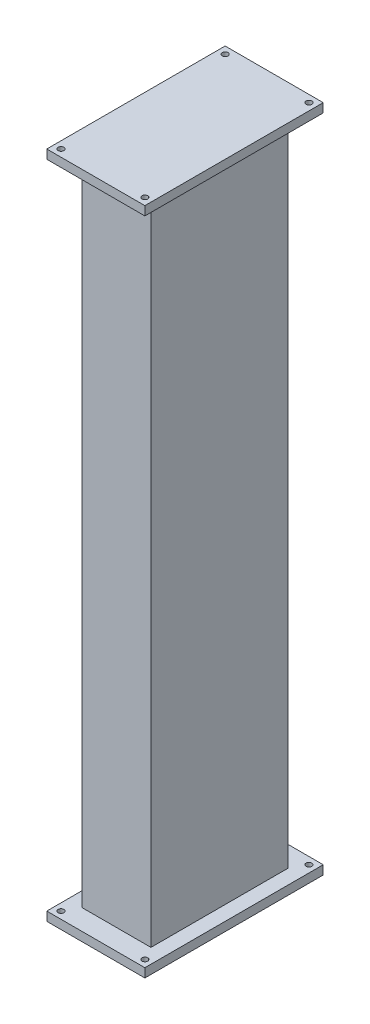
from build123d import *

# Parameters (mm, degrees)
SKETCH1_W           = 110
SKETCH1_H           = 200
SKETCH1_R           = 3.25
BOSS_EXTRUDE1_DEPTH = 10
SKETCH2_W           = 77.344894784
SKETCH2_H           = 153.75567248
BOSS_EXTRUDE2_DEPTH = 730
SKETCH4_W           = 110
SKETCH4_H           = 200
SKETCH4_R           = 3.25
BOSS_EXTRUDE4_DEPTH = 10


with BuildPart() as part:
    # Sketch1 → Boss-Extrude1 (new body)
    with BuildSketch(Plane(origin=(0, 0, 0), x_dir=(1, 0, 0), z_dir=(0, 1, 0))):
        Rectangle(SKETCH1_W, SKETCH1_H)
        with Locations(Location((-47, 92, 0), (0, 0, 270))):
            Circle(SKETCH1_R, mode=Mode.SUBTRACT)
        with Locations(Location((47, 92, 0), (0, 0, 270))):
            Circle(SKETCH1_R, mode=Mode.SUBTRACT)
        with Locations(Location((47, -92, 0), (0, 0, 270))):
            Circle(SKETCH1_R, mode=Mode.SUBTRACT)
        with Locations(Location((-47, -92, 0), (0, 0, 270))):
            Circle(SKETCH1_R, mode=Mode.SUBTRACT)
    extrude(amount=BOSS_EXTRUDE1_DEPTH)

    # Sketch2 → Boss-Extrude2 (add)
    with BuildSketch(Plane(origin=(0, 10, 0), x_dir=(1, 0, 0), z_dir=(0, 1, 0))):
        Rectangle(SKETCH2_W, SKETCH2_H)
    extrude(amount=BOSS_EXTRUDE2_DEPTH)

    # Sketch4 → Boss-Extrude4 (add)
    with BuildSketch(Plane(origin=(0, 740, 0), x_dir=(1, 0, 0), z_dir=(0, 1, 0))):
        Rectangle(SKETCH4_W, SKETCH4_H)
        with Locations(Location((-47, 92, 0), (0, 0, 270))):
            Circle(SKETCH4_R, mode=Mode.SUBTRACT)
        with Locations(Location((47, 92, 0), (0, 0, 270))):
            Circle(SKETCH4_R, mode=Mode.SUBTRACT)
        with Locations(Location((47, -92, 0), (0, 0, 270))):
            Circle(SKETCH4_R, mode=Mode.SUBTRACT)
        with Locations(Location((-47, -92, 0), (0, 0, 270))):
            Circle(SKETCH4_R, mode=Mode.SUBTRACT)
    extrude(amount=BOSS_EXTRUDE4_DEPTH)


solid = part.part
